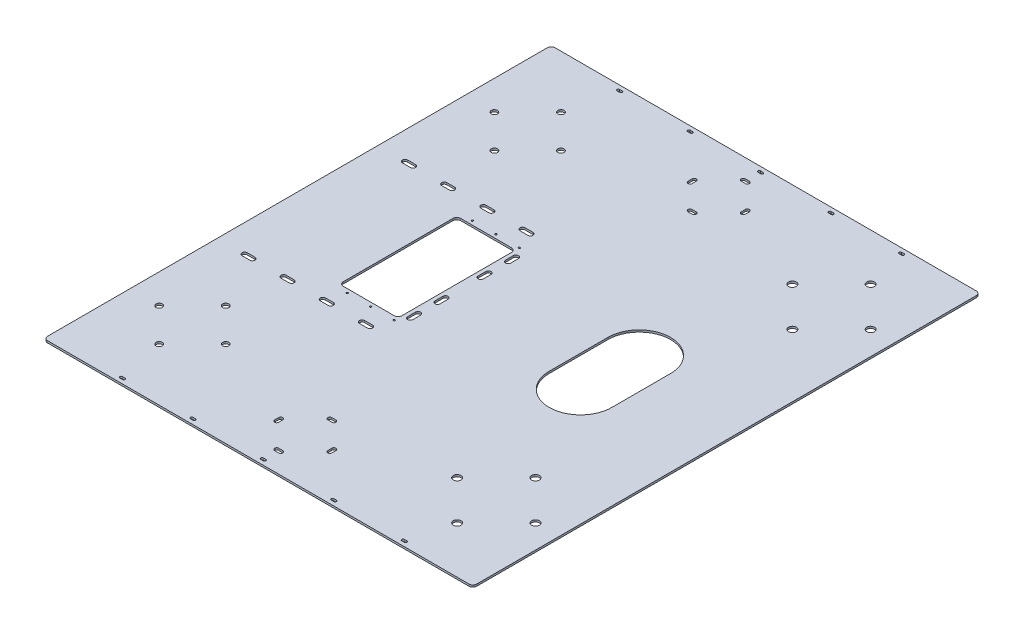
from build123d import *

# Parameters (mm, degrees)
SKETCH_1_W             = 1096
SKETCH_1_H             = 1296
EXTRUDE_1_DEPTH        = 5
CUT_EXTRUDE_1_DEPTH    = 10
CUT_EXTRUDE_2_DEPTH    = 10
PATTERN_LINEAR_1_COUNT = 4
PATTERN_LINEAR_1_PITCH = 100
CUT_EXTRUDE_3_DEPTH    = 10
PATTERN_LINEAR_2_COUNT = 2
PATTERN_LINEAR_2_PITCH = 70
SKETCH_5_R             = 10
CUT_EXTRUDE_4_DEPTH    = 10
SKETCH_6_R             = 8
CUT_EXTRUDE_5_DEPTH    = 10
MIRROR_1_COPY_1_DEPTH  = 10
MIRROR_1_COPY_2_DEPTH  = 10
MIRROR_1_COPY_3_DEPTH  = 10
MIRROR_1_COPY_4_DEPTH  = 10
SKETCH_7_W             = 150
SKETCH_7_H             = 300
CUT_EXTRUDE_6_DEPTH    = 10
CUT_EXTRUDE_7_DEPTH    = 10
FILLET_1_R             = 10
PATTERN_LINEAR_3_COUNT = 5
PATTERN_LINEAR_3_PITCH = 180
MIRROR_3_COPY_1_DEPTH  = 10
MIRROR_3_COPY_2_DEPTH  = 10
MIRROR_3_COPY_3_DEPTH  = 10
MIRROR_3_COPY_4_DEPTH  = 10
CUT_EXTRUDE_8_DEPTH    = 10
SKETCH_10_R            = 2.2
CUT_EXTRUDE_9_DEPTH    = 102
FILLET_2_R             = 10


with BuildPart() as part:
    # 草图1 → 凸台-拉伸1 (new body)
    with BuildSketch(Plane(origin=(0, 0, 0), x_dir=(1, 0, 0), z_dir=(0, 1, 0))):
        Rectangle(SKETCH_1_W, SKETCH_1_H)
    extrude(amount=EXTRUDE_1_DEPTH)

    # 草图2 → 切除-拉伸1 (cut)
    with BuildSketch(Plane.XZ):
        with BuildLine():
            ThreePointArc((5.651115561, 601.031687595), (0, 601.25), (-5.651115561, 601.031687595))
            ThreePointArc((-5.651115561, 601.031687595), (-10.480439836, 595.392305798), (-4.84105804, 590.562981523))
            ThreePointArc((-4.84105804, 590.562981523), (0, 590.75), (4.84105804, 590.562981523))
            ThreePointArc((4.84105804, 590.562981523), (10.480439836, 595.392305798), (5.651115561, 601.031687595))
        make_face()
        with BuildLine():
            ThreePointArc((73.031687595, 522.348884439), (73.25, 528), (73.031687595, 533.651115561))
            ThreePointArc((73.031687595, 533.651115561), (67.392305798, 538.480439836), (62.562981523, 532.84105804))
            ThreePointArc((62.562981523, 532.84105804), (62.75, 528), (62.562981523, 523.15894196))
            ThreePointArc((62.562981523, 523.15894196), (67.392305798, 517.519560164), (73.031687595, 522.348884439))
        make_face()
        with BuildLine():
            ThreePointArc((-5.651115561, 454.968312405), (0, 454.75), (5.651115561, 454.968312405))
            ThreePointArc((5.651115561, 454.968312405), (10.480439836, 460.607694202), (4.84105804, 465.437018477))
            ThreePointArc((4.84105804, 465.437018477), (0, 465.25), (-4.84105804, 465.437018477))
            ThreePointArc((-4.84105804, 465.437018477), (-10.480439836, 460.607694202), (-5.651115561, 454.968312405))
        make_face()
        with BuildLine():
            ThreePointArc((-73.031687595, 533.651115561), (-73.25, 528), (-73.031687595, 522.348884439))
            ThreePointArc((-73.031687595, 522.348884439), (-67.392305798, 517.519560164), (-62.562981523, 523.15894196))
            ThreePointArc((-62.562981523, 523.15894196), (-62.75, 528), (-62.562981523, 532.84105804))
            ThreePointArc((-62.562981523, 532.84105804), (-67.392305798, 538.480439836), (-73.031687595, 533.651115561))
        make_face()
    cut_extrude_1 = extrude(amount=-CUT_EXTRUDE_1_DEPTH, mode=Mode.SUBTRACT)

    # 草图3 → 切除-拉伸2 (cut)
    with BuildSketch(Plane(origin=(0, 5, 0), x_dir=(1, 0, 0), z_dir=(0, 1, 0))):
        with BuildLine():
            Line((-178, -198.4), (-158, -198.4))
            ThreePointArc((-158, -198.4), (-151.4, -205), (-158, -211.6))
            Line((-158, -211.6), (-178, -211.6))
            ThreePointArc((-178, -211.6), (-184.6, -205), (-178, -198.4))
        make_face()
    cut_extrude_2 = extrude(amount=-CUT_EXTRUDE_2_DEPTH, mode=Mode.SUBTRACT)

    # 阵列(线性)1: 切除-拉伸2 ×4
    with Locations(*[(-i * PATTERN_LINEAR_1_PITCH, 0, 0) for i in range(1, PATTERN_LINEAR_1_COUNT)]):
        add(cut_extrude_2, mode=Mode.SUBTRACT)

    # 镜向2: 切除-拉伸1 across plane
    add(cut_extrude_1.mirror(Plane.XY), mode=Mode.SUBTRACT)

    # 草图4 → 切除-拉伸3 (cut)
    with BuildSketch(Plane(origin=(0, 5, 0), x_dir=(1, 0, 0), z_dir=(0, 1, 0))):
        with BuildLine():
            Line((-118.4, 135), (-118.4, 115))
            ThreePointArc((-118.4, 115), (-125, 108.4), (-131.6, 115))
            Line((-131.6, 115), (-131.6, 135))
            ThreePointArc((-131.6, 135), (-125, 141.6), (-118.4, 135))
        make_face()
    cut_extrude_3 = extrude(amount=-CUT_EXTRUDE_3_DEPTH, mode=Mode.SUBTRACT)

    # 阵列(线性)2: 切除-拉伸3 ×2
    with Locations(*[(0, 0, i * PATTERN_LINEAR_2_PITCH) for i in range(1, PATTERN_LINEAR_2_COUNT)]):
        add(cut_extrude_3, mode=Mode.SUBTRACT)

    # 草图5 → 切除-拉伸4 (cut)
    with BuildSketch(Plane.XZ):
        with Locations(Location((488, -428, 0), (0, 0, 270))):
            Circle(SKETCH_5_R)
        with Locations(Location((388, -528, 0), (0, 0, 270))):
            Circle(SKETCH_5_R)
        with Locations(Location((288, -428, 0), (0, 0, 270))):
            Circle(SKETCH_5_R)
        with Locations(Location((388, -328, 0), (0, 0, 270))):
            Circle(SKETCH_5_R)
    cut_extrude_4 = extrude(amount=-CUT_EXTRUDE_4_DEPTH, mode=Mode.SUBTRACT)

    # 草图6 → 切除-拉伸5 (cut)
    with BuildSketch(Plane.XZ):
        with Locations(Location((-303, -428, 0), (0, 0, 270))):
            Circle(SKETCH_6_R)
        with Locations(Location((-388, -513, 0), (0, 0, 270))):
            Circle(SKETCH_6_R)
        with Locations(Location((-473, -428, 0), (0, 0, 270))):
            Circle(SKETCH_6_R)
        with Locations(Location((-388, -343, 0), (0, 0, 270))):
            Circle(SKETCH_6_R)
    cut_extrude_5 = extrude(amount=-CUT_EXTRUDE_5_DEPTH, mode=Mode.SUBTRACT)

    # 镜向1: 切除-拉伸2, 切除-拉伸3, 切除-拉伸4, 切除-拉伸5 across plane
    add(cut_extrude_2.mirror(Plane.XY), mode=Mode.SUBTRACT)
    add(cut_extrude_3.mirror(Plane.XY), mode=Mode.SUBTRACT)
    add(cut_extrude_4.mirror(Plane.XY), mode=Mode.SUBTRACT)
    add(cut_extrude_5.mirror(Plane.XY), mode=Mode.SUBTRACT)

    # 镜向1 copy 1 sketch → 镜向1 copy 1 (cut)
    with BuildSketch(Plane(origin=(-100, 5, 0), x_dir=(1, 0, 0), z_dir=(0, 1, 0))):
        with BuildLine():
            Line((-178, 198.4), (-158, 198.4))
            ThreePointArc((-158, 198.4), (-151.4, 205), (-158, 211.6))
            Line((-158, 211.6), (-178, 211.6))
            ThreePointArc((-178, 211.6), (-184.6, 205), (-178, 198.4))
        make_face()
    extrude(amount=-MIRROR_1_COPY_1_DEPTH, mode=Mode.SUBTRACT)

    # 镜向1 copy 2 sketch → 镜向1 copy 2 (cut)
    with BuildSketch(Plane(origin=(-200, 5, 0), x_dir=(1, 0, 0), z_dir=(0, 1, 0))):
        with BuildLine():
            Line((-178, 198.4), (-158, 198.4))
            ThreePointArc((-158, 198.4), (-151.4, 205), (-158, 211.6))
            Line((-158, 211.6), (-178, 211.6))
            ThreePointArc((-178, 211.6), (-184.6, 205), (-178, 198.4))
        make_face()
    extrude(amount=-MIRROR_1_COPY_2_DEPTH, mode=Mode.SUBTRACT)

    # 镜向1 copy 3 sketch → 镜向1 copy 3 (cut)
    with BuildSketch(Plane(origin=(-300, 5, 0), x_dir=(1, 0, 0), z_dir=(0, 1, 0))):
        with BuildLine():
            Line((-178, 198.4), (-158, 198.4))
            ThreePointArc((-158, 198.4), (-151.4, 205), (-158, 211.6))
            Line((-158, 211.6), (-178, 211.6))
            ThreePointArc((-178, 211.6), (-184.6, 205), (-178, 198.4))
        make_face()
    extrude(amount=-MIRROR_1_COPY_3_DEPTH, mode=Mode.SUBTRACT)

    # 镜向1 copy 4 sketch → 镜向1 copy 4 (cut)
    with BuildSketch(Plane(origin=(0, 5, -70), x_dir=(1, 0, 0), z_dir=(0, 1, 0))):
        with BuildLine():
            Line((-118.4, -135), (-118.4, -115))
            ThreePointArc((-118.4, -115), (-125, -108.4), (-131.6, -115))
            Line((-131.6, -115), (-131.6, -135))
            ThreePointArc((-131.6, -135), (-125, -141.6), (-118.4, -135))
        make_face()
    extrude(amount=-MIRROR_1_COPY_4_DEPTH, mode=Mode.SUBTRACT)

    # 草图7 → 切除-拉伸6 (cut)
    with BuildSketch(Plane.XZ):
        with Locations((-216, 0)):
            Rectangle(SKETCH_7_W, SKETCH_7_H)
    extrude(amount=-CUT_EXTRUDE_6_DEPTH, mode=Mode.SUBTRACT)

    # 草图8 → 切除-拉伸7 (cut)
    with BuildSketch(Plane.XZ):
        with BuildLine():
            Line((-356.7, 631.7), (-363.3, 631.7))
            ThreePointArc((-363.3, 631.7), (-366.6, 635), (-363.3, 638.3))
            Line((-363.3, 638.3), (-356.7, 638.3))
            ThreePointArc((-356.7, 638.3), (-353.4, 635), (-356.7, 631.7))
        make_face()
    cut_extrude_7 = extrude(amount=-CUT_EXTRUDE_7_DEPTH, mode=Mode.SUBTRACT)

    # 圆角1
    fillet_1_edges = [part.edges().sort_by_distance(p)[0] for p in [
        (-291, 2.5, -150),
        (-291, 2.5, 150),
        (-141, 2.5, 150),
        (-141, 2.5, -150),
    ]]
    fillet(fillet_1_edges, radius=FILLET_1_R)

    # 阵列(线性)3: 切除-拉伸7 ×5
    with Locations(*[(i * PATTERN_LINEAR_3_PITCH, 0, 0) for i in range(1, PATTERN_LINEAR_3_COUNT)]):
        add(cut_extrude_7, mode=Mode.SUBTRACT)

    # 镜向3: 切除-拉伸7 across plane
    add(cut_extrude_7.mirror(Plane.XY), mode=Mode.SUBTRACT)

    # 镜向3 copy 1 sketch → 镜向3 copy 1 (cut)
    with BuildSketch(Plane(origin=(180, 0, 0), x_dir=(1, 0, 0), z_dir=(0, -1, 0))):
        with BuildLine():
            Line((-356.7, -631.7), (-363.3, -631.7))
            ThreePointArc((-363.3, -631.7), (-366.6, -635), (-363.3, -638.3))
            Line((-363.3, -638.3), (-356.7, -638.3))
            ThreePointArc((-356.7, -638.3), (-353.4, -635), (-356.7, -631.7))
        make_face()
    extrude(amount=-MIRROR_3_COPY_1_DEPTH, mode=Mode.SUBTRACT)

    # 镜向3 copy 2 sketch → 镜向3 copy 2 (cut)
    with BuildSketch(Plane(origin=(360, 0, 0), x_dir=(1, 0, 0), z_dir=(0, -1, 0))):
        with BuildLine():
            Line((-356.7, -631.7), (-363.3, -631.7))
            ThreePointArc((-363.3, -631.7), (-366.6, -635), (-363.3, -638.3))
            Line((-363.3, -638.3), (-356.7, -638.3))
            ThreePointArc((-356.7, -638.3), (-353.4, -635), (-356.7, -631.7))
        make_face()
    extrude(amount=-MIRROR_3_COPY_2_DEPTH, mode=Mode.SUBTRACT)

    # 镜向3 copy 3 sketch → 镜向3 copy 3 (cut)
    with BuildSketch(Plane(origin=(540, 0, 0), x_dir=(1, 0, 0), z_dir=(0, -1, 0))):
        with BuildLine():
            Line((-356.7, -631.7), (-363.3, -631.7))
            ThreePointArc((-363.3, -631.7), (-366.6, -635), (-363.3, -638.3))
            Line((-363.3, -638.3), (-356.7, -638.3))
            ThreePointArc((-356.7, -638.3), (-353.4, -635), (-356.7, -631.7))
        make_face()
    extrude(amount=-MIRROR_3_COPY_3_DEPTH, mode=Mode.SUBTRACT)

    # 镜向3 copy 4 sketch → 镜向3 copy 4 (cut)
    with BuildSketch(Plane(origin=(720, 0, 0), x_dir=(1, 0, 0), z_dir=(0, -1, 0))):
        with BuildLine():
            Line((-356.7, -631.7), (-363.3, -631.7))
            ThreePointArc((-363.3, -631.7), (-366.6, -635), (-363.3, -638.3))
            Line((-363.3, -638.3), (-356.7, -638.3))
            ThreePointArc((-356.7, -638.3), (-353.4, -635), (-356.7, -631.7))
        make_face()
    extrude(amount=-MIRROR_3_COPY_4_DEPTH, mode=Mode.SUBTRACT)

    # 草图9 → 切除-拉伸8 (cut)
    with BuildSketch(Plane.XZ):
        with BuildLine():
            Line((170, -75), (170, 75))
            ThreePointArc((170, 75), (250, 155), (330, 75))
            Line((330, 75), (330, -75))
            ThreePointArc((330, -75), (250, -155), (170, -75))
        make_face()
    extrude(amount=-CUT_EXTRUDE_8_DEPTH, mode=Mode.SUBTRACT)

    # 草图10 → 切除-拉伸9 (cut)
    with BuildSketch(Plane.XZ):
        with Locations(Location((-141, 160, 0), (0, 0, 270))):
            Circle(SKETCH_10_R)
        with Locations(Location((-201, 160, 0), (0, 0, 270))):
            Circle(SKETCH_10_R)
        with Locations(Location((-261, 160, 0), (0, 0, 270))):
            Circle(SKETCH_10_R)
    cut_extrude_9 = extrude(amount=-CUT_EXTRUDE_9_DEPTH, mode=Mode.SUBTRACT)

    # 镜向4: 切除-拉伸9 across plane
    add(cut_extrude_9.mirror(Plane.XY), mode=Mode.SUBTRACT)

    # 圆角2
    fillet_2_edges = [part.edges().sort_by_distance(p)[0] for p in [
        (-548, 2.5, -648),
        (548, 2.5, -648),
        (548, 2.5, 648),
        (-548, 2.5, 648),
    ]]
    fillet(fillet_2_edges, radius=FILLET_2_R)


solid = part.part
